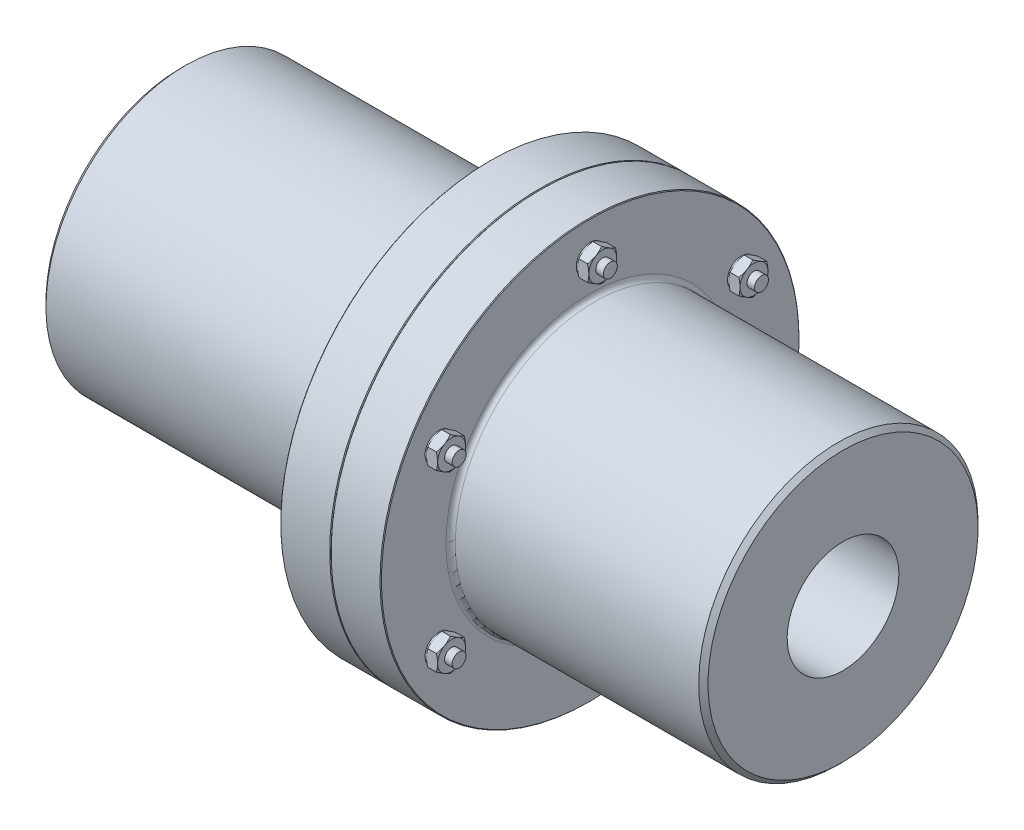
from build123d import *

# Parameters (mm, degrees)
CHAMFER1_SIZE                   = 3.333333333
CHAMFER2_SIZE                   = 0.5
FILLET1_R                       = 1
SKETCH15_R                      = 65
CUT_EXTRUDE5_DEPTH              = 334.240153643
CUT_EXTRUDE7_DEPTH              = 334.240153643
SKETCH16_R                      = 60
CUT_EXTRUDE6_DEPTH              = 334.240153643
CHAMFER3_SIZE                   = 0.5
CHAMFER4_SIZE                   = 3.333333333
FILLET2_R                       = 3.333333333
SKETCH6_R                       = 5
CUT_EXTRUDE1_DEPTH              = 72
CHAMFER5_SIZE                   = 0.2
CHAMFER6_SIZE                   = 0.2
CIRCPATTERN1_COUNT              = 6
CHAMFER5_OF_CIRCPATTERN1_SIZE   = 0.2
CHAMFER6_OF_CIRCPATTERN1_SIZE   = 0.2
SKETCH7_W                       = 86.4
SKETCH7_H                       = 5
BOSS_EXTRUDE1_DEPTH             = 8
SKETCH9_R                       = 15
SKETCH9_R_2                     = 10
CUT_EXTRUDE2_DEPTH              = 1
CUT_EXTRUDE2_DRAFT              = -60
SKETCH10_R                      = 10
BOSS_EXTRUDE2_DEPTH             = 1
BOSS_EXTRUDE3_DEPTH             = 8
SKETCH12_R                      = 15
SKETCH12_R_2                    = 10
CUT_EXTRUDE3_DEPTH              = 1
CUT_EXTRUDE3_DRAFT              = -60
SKETCH13_R                      = 15
SKETCH13_R_2                    = 10
CUT_EXTRUDE4_DEPTH              = 1
CUT_EXTRUDE4_DRAFT              = -60
CIRCPATTERN3_COUNT              = 6
CIRCPATTERN3_COPY_1_SKETCH_R    = 15
CIRCPATTERN3_COPY_1_SKETCH_R_2  = 10
CIRCPATTERN3_COPY_1_DEPTH       = 1
CIRCPATTERN3_COPY_1_DRAFT       = -60
CIRCPATTERN3_COPY_2_SKETCH_R    = 15
CIRCPATTERN3_COPY_2_SKETCH_R_2  = 10
CIRCPATTERN3_COPY_2_DEPTH       = 1
CIRCPATTERN3_COPY_2_DRAFT       = -60
CIRCPATTERN3_COPY_3_SKETCH_R    = 15
CIRCPATTERN3_COPY_3_SKETCH_R_2  = 10
CIRCPATTERN3_COPY_3_DEPTH       = 1
CIRCPATTERN3_COPY_3_DRAFT       = -60
CIRCPATTERN3_COPY_4_SKETCH_R    = 15
CIRCPATTERN3_COPY_4_SKETCH_R_2  = 10
CIRCPATTERN3_COPY_4_DEPTH       = 1
CIRCPATTERN3_COPY_4_DRAFT       = -60
CIRCPATTERN3_COPY_5_SKETCH_R    = 15
CIRCPATTERN3_COPY_5_SKETCH_R_2  = 10
CIRCPATTERN3_COPY_5_DEPTH       = 1
CIRCPATTERN3_COPY_5_DRAFT       = -60
CIRCPATTERN3_COPY_6_SKETCH_R    = 15
CIRCPATTERN3_COPY_6_SKETCH_R_2  = 10
CIRCPATTERN3_COPY_6_DEPTH       = 1
CIRCPATTERN3_COPY_6_DRAFT       = -60
CIRCPATTERN3_COPY_7_SKETCH_R    = 15
CIRCPATTERN3_COPY_7_SKETCH_R_2  = 10
CIRCPATTERN3_COPY_7_DEPTH       = 1
CIRCPATTERN3_COPY_7_DRAFT       = -60
CIRCPATTERN3_COPY_8_SKETCH_R    = 15
CIRCPATTERN3_COPY_8_SKETCH_R_2  = 10
CIRCPATTERN3_COPY_8_DEPTH       = 1
CIRCPATTERN3_COPY_8_DRAFT       = -60
CIRCPATTERN3_COPY_9_SKETCH_R    = 15
CIRCPATTERN3_COPY_9_SKETCH_R_2  = 10
CIRCPATTERN3_COPY_9_DEPTH       = 1
CIRCPATTERN3_COPY_9_DRAFT       = -60
CIRCPATTERN3_COPY_10_SKETCH_R   = 15
CIRCPATTERN3_COPY_10_SKETCH_R_2 = 10
CIRCPATTERN3_COPY_10_DEPTH      = 1
CIRCPATTERN3_COPY_10_DRAFT      = -60
CIRCPATTERN3_COPY_11_SKETCH_R   = 15
CIRCPATTERN3_COPY_11_SKETCH_R_2 = 10
CIRCPATTERN3_COPY_11_DEPTH      = 1
CIRCPATTERN3_COPY_11_DRAFT      = -60
CIRCPATTERN3_COPY_12_SKETCH_R   = 15
CIRCPATTERN3_COPY_12_SKETCH_R_2 = 10
CIRCPATTERN3_COPY_12_DEPTH      = 1
CIRCPATTERN3_COPY_12_DRAFT      = -60
CIRCPATTERN3_COPY_13_SKETCH_R   = 15
CIRCPATTERN3_COPY_13_SKETCH_R_2 = 10
CIRCPATTERN3_COPY_13_DEPTH      = 1
CIRCPATTERN3_COPY_13_DRAFT      = -60
CIRCPATTERN3_COPY_14_SKETCH_R   = 15
CIRCPATTERN3_COPY_14_SKETCH_R_2 = 10
CIRCPATTERN3_COPY_14_DEPTH      = 1
CIRCPATTERN3_COPY_14_DRAFT      = -60
CIRCPATTERN3_COPY_15_SKETCH_R   = 15
CIRCPATTERN3_COPY_15_SKETCH_R_2 = 10
CIRCPATTERN3_COPY_15_DEPTH      = 1
CIRCPATTERN3_COPY_15_DRAFT      = -60
SKETCH27_R                      = 60
SKETCH27_R_2                    = 40
BOSS_EXTRUDE4_DEPTH             = 212


with BuildPart() as part:
    # Sketch2 → Revolve1 (revolve)
    with BuildSketch(Plane.XY, mode=Mode.PRIVATE) as revolve1_sk:
        Polygon((-257, 100), (-257, 0), (-5, 0), (-5, 105), (0, 105), (0, 150), (-36, 150), (-36, 100), align=None)
    revolve(revolve1_sk.sketch.rotate(Axis((-257, 0, 0), (1, 0, 0)), 180), axis=Axis((-257, 0, 0), (1, 0, 0)))

    # Chamfer1
    chamfer1_edges = [part.edges().sort_by_distance(p)[0] for p in [
        (-257, 100, 0),
    ]]
    chamfer(chamfer1_edges, length=CHAMFER1_SIZE)

    # Chamfer2
    chamfer2_edges = [part.edges().sort_by_distance(p)[0] for p in [
        (-36, 150, 0),
        (0, 150, 0),
    ]]
    chamfer(chamfer2_edges, length=CHAMFER2_SIZE)

    # Fillet1
    fillet1_edges = [part.edges().sort_by_distance(p)[0] for p in [
        (-36, 100, 0),
    ]]
    fillet(fillet1_edges, radius=FILLET1_R)

    # Sketch15 → Cut-Extrude5 (cut, through all)
    with BuildSketch(Plane(origin=(0, 0, 0), x_dir=(0, 0, -1), z_dir=(1, 0, 0))):
        Circle(SKETCH15_R)
    extrude(amount=-CUT_EXTRUDE5_DEPTH, mode=Mode.SUBTRACT)

    # Sketch20 → Cut-Extrude7 (cut, through all)
    with BuildSketch(Plane(origin=(0, 0, 0), x_dir=(0, 0, -1), z_dir=(1, 0, 0))):
        with BuildLine():
            Line((72.4, -16), (72.4, 16))
            Line((72.4, 16), (63, 16))
            ThreePointArc((63, 16), (64.498061986, 8.062257748), (65, 0))
            ThreePointArc((65, 0), (64.498061986, -8.062257748), (63, -16))
            Line((63, -16), (72.4, -16))
        make_face()
    extrude(amount=-CUT_EXTRUDE7_DEPTH, mode=Mode.SUBTRACT)


with BuildPart() as body_2:
    # Sketch3 → Revolve2 (revolve)
    with BuildSketch(Plane.XY):
        Polygon((36, 150), (0, 150), (0, 105), (5, 105), (5, 0), (217, 0), (217, 60), (217, 100), (36, 100), align=None)
    revolve(axis=Axis((-257, 0, 0), (1, 0, 0)))

    # Sketch16 → Cut-Extrude6 (cut, through all)
    with BuildSketch(Plane(origin=(0, 0, 0), x_dir=(0, 0, -1), z_dir=(1, 0, 0))):
        with Locations(Location((0, 0, 0), (0, 0, 90))):
            Circle(SKETCH16_R)
    extrude(amount=CUT_EXTRUDE6_DEPTH, mode=Mode.SUBTRACT)

    # Chamfer3
    chamfer3_edges = [body_2.edges().sort_by_distance(p)[0] for p in [
        (36, -150, 0),
        (0, -150, 0),
    ]]
    chamfer(chamfer3_edges, length=CHAMFER3_SIZE)

    # Chamfer4
    chamfer4_edges = [body_2.edges().sort_by_distance(p)[0] for p in [
        (217, -100, 0),
    ]]
    chamfer(chamfer4_edges, length=CHAMFER4_SIZE)

    # Fillet2
    fillet2_edges = [body_2.edges().sort_by_distance(p)[0] for p in [
        (36, -100, 0),
    ]]
    fillet(fillet2_edges, radius=FILLET2_R)


with BuildPart() as cut_extrude1_tool:
    # Sketch6 → Cut-Extrude1 (new body)
    with BuildSketch(Plane.ZY.offset(36)):
        with Locations((0, 125)):
            Circle(SKETCH6_R)
    cut_extrude1 = extrude(amount=-CUT_EXTRUDE1_DEPTH)


with BuildPart() as part_1:
    add(part.part)

    # Cut-Extrude1: cut by cut_extrude1_tool
    add(cut_extrude1_tool.part, mode=Mode.SUBTRACT)

    # Chamfer5
    chamfer5_edges = [part_1.edges().sort_by_distance(p)[0] for p in [
        (-36, 125, -5),
    ]]
    chamfer(chamfer5_edges, length=CHAMFER5_SIZE)


with BuildPart() as body_2_1:
    add(body_2.part)

    # Cut-Extrude1: cut by cut_extrude1_tool
    add(cut_extrude1_tool.part, mode=Mode.SUBTRACT)

    # Chamfer6
    chamfer6_edges = [body_2_1.edges().sort_by_distance(p)[0] for p in [
        (36, 125, -5),
    ]]
    chamfer(chamfer6_edges, length=CHAMFER6_SIZE)


with BuildPart() as circpattern1_tool:
    # CircPattern1: Cut-Extrude1 ×6 about axis
    circpattern1_axis = Axis((0, 0, 0), (1, 0, 0))
    for i in range(1, CIRCPATTERN1_COUNT):
        add(cut_extrude1.rotate(circpattern1_axis, i * 360 / CIRCPATTERN1_COUNT))


with BuildPart() as part_2:
    add(part_1.part)

    # CircPattern1: cut by circpattern1_tool
    add(circpattern1_tool.part, mode=Mode.SUBTRACT)

    # Chamfer5 of CircPattern1
    chamfer5_of_circpattern1_edges = [part_2.edges().sort_by_distance(p)[0] for p in [
        (-36, 66.830127019, 105.753175473),
        (-36, -58.169872981, 110.753175473),
        (-36, -125, 5),
        (-36, -66.830127019, -105.753175473),
        (-36, 58.169872981, -110.753175473),
    ]]
    chamfer(chamfer5_of_circpattern1_edges, length=CHAMFER5_OF_CIRCPATTERN1_SIZE)



with BuildPart() as body_2_2:
    add(body_2_1.part)

    # CircPattern1: cut by circpattern1_tool
    add(circpattern1_tool.part, mode=Mode.SUBTRACT)

    # Chamfer6 of CircPattern1
    chamfer6_of_circpattern1_edges = [body_2_2.edges().sort_by_distance(p)[0] for p in [
        (36, 66.830127019, 105.753175473),
        (36, -58.169872981, 110.753175473),
        (36, -125, 5),
        (36, -66.830127019, -105.753175473),
        (36, 58.169872981, -110.753175473),
    ]]
    chamfer(chamfer6_of_circpattern1_edges, length=CHAMFER6_OF_CIRCPATTERN1_SIZE)


with BuildPart() as part_3:
    add(part_2.part)

    add(body_2_2.part)  # Revolve3 merges body 2
    # Sketch7 → Revolve3 (revolve)
    with BuildSketch(Plane.XY, mode=Mode.PRIVATE) as revolve3_sk:
        with Locations((7.2, 127.5)):
            Rectangle(SKETCH7_W, SKETCH7_H)
    revolve3 = revolve(revolve3_sk.sketch.rotate(Axis((50.4, 125, 0), (-1, 0, 0)), 90), axis=Axis((50.4, 125, 0), (-1, 0, 0)))

    # Sketch8 → Boss-Extrude1 (add)
    with BuildSketch(Plane.ZY.offset(36)):
        Polygon((0, 136.547005384), (-10, 130.773502692), (-10, 119.226497308), (0, 113.452994616), (10, 119.226497308), (10, 130.773502692), align=None)
    boss_extrude1 = extrude(amount=BOSS_EXTRUDE1_DEPTH)


with BuildPart() as cut_extrude2_tool:
    # Sketch9 → Cut-Extrude2 (with draft: the straight prism first)
    with BuildSketch(Plane.ZY.offset(44)):
        with Locations((0, 125)):
            Circle(SKETCH9_R)
        with Locations((0, 125)):
            Circle(SKETCH9_R_2, mode=Mode.SUBTRACT)
    extrude(amount=-CUT_EXTRUDE2_DEPTH)
    # Cut-Extrude2: the draft: its side faces are tilted about the plane it starts from
    cut_extrude2_sides = [cut_extrude2_tool.faces().sort_by_distance(p)[0] for p in [
        (-43.5, 125, -15),
        (-43.5, 125, -10),
    ]]
    draft(cut_extrude2_sides, Plane.ZY.offset(44), CUT_EXTRUDE2_DRAFT)


with BuildPart() as part_4:
    add(part_3.part)

    # Cut-Extrude2: cut by cut_extrude2_tool
    add(cut_extrude2_tool.part, mode=Mode.SUBTRACT)

    # Sketch10 → Boss-Extrude2 (add)
    with BuildSketch(Plane(origin=(36, 0, 0), x_dir=(0, 0, -1), z_dir=(1, 0, 0))):
        with Locations(Location((0, 125, 0), (0, 0, 270))):
            Circle(SKETCH10_R)
    boss_extrude2 = extrude(amount=BOSS_EXTRUDE2_DEPTH)

    # Sketch11 → Boss-Extrude3 (add)
    with BuildSketch(Plane(origin=(37, 0, 0), x_dir=(0, 0, -1), z_dir=(1, 0, 0))):
        Polygon((10, 130.773502692), (0, 136.547005384), (-10, 130.773502692), (-10, 119.226497308), (0, 113.452994616), (10, 119.226497308), align=None)
    boss_extrude3 = extrude(amount=BOSS_EXTRUDE3_DEPTH)


with BuildPart() as cut_extrude3_tool:
    # Sketch12 → Cut-Extrude3 (with draft: the straight prism first)
    with BuildSketch(Plane(origin=(45, 0, 0), x_dir=(0, 0, -1), z_dir=(1, 0, 0))):
        with Locations((0, 125)):
            Circle(SKETCH12_R)
        with Locations(Location((0, 125, 0), (0, 0, 180))):
            Circle(SKETCH12_R_2, mode=Mode.SUBTRACT)
    extrude(amount=-CUT_EXTRUDE3_DEPTH)
    # Cut-Extrude3: the draft: its side faces are tilted about the plane it starts from
    cut_extrude3_sides = [cut_extrude3_tool.faces().sort_by_distance(p)[0] for p in [
        (44.5, 125, 15),
        (44.5, 125, -10),
    ]]
    draft(cut_extrude3_sides, Plane(origin=(45, 0, 0), x_dir=(0, 0, -1), z_dir=(1, 0, 0)), CUT_EXTRUDE3_DRAFT)


with BuildPart() as part_5:
    add(part_4.part)

    # Cut-Extrude3: cut by cut_extrude3_tool
    add(cut_extrude3_tool.part, mode=Mode.SUBTRACT)


with BuildPart() as cut_extrude4_tool:
    # Sketch13 → Cut-Extrude4 (with draft: the straight prism first)
    with BuildSketch(Plane.ZY.offset(-37)):
        with Locations((0, 125)):
            Circle(SKETCH13_R)
        with Locations((0, 125)):
            Circle(SKETCH13_R_2, mode=Mode.SUBTRACT)
    extrude(amount=-CUT_EXTRUDE4_DEPTH)
    # Cut-Extrude4: the draft: its side faces are tilted about the plane it starts from
    cut_extrude4_sides = [cut_extrude4_tool.faces().sort_by_distance(p)[0] for p in [
        (37.5, 125, -15),
        (37.5, 125, -10),
    ]]
    draft(cut_extrude4_sides, Plane.ZY.offset(-37), CUT_EXTRUDE4_DRAFT)


with BuildPart() as part_6:
    add(part_5.part)

    # Cut-Extrude4: cut by cut_extrude4_tool
    add(cut_extrude4_tool.part, mode=Mode.SUBTRACT)

    # CircPattern3: Revolve3, Boss-Extrude1, Boss-Extrude2, Boss-Extrude3 ×6 about axis
    circpattern3_axis = Axis((0, 0, 0), (1, 0, 0))
    add([revolve3.rotate(circpattern3_axis, i * 360 / CIRCPATTERN3_COUNT) for i in range(1, CIRCPATTERN3_COUNT)])
    add([boss_extrude1.rotate(circpattern3_axis, i * 360 / CIRCPATTERN3_COUNT) for i in range(1, CIRCPATTERN3_COUNT)])
    add([boss_extrude2.rotate(circpattern3_axis, i * 360 / CIRCPATTERN3_COUNT) for i in range(1, CIRCPATTERN3_COUNT)])
    add([boss_extrude3.rotate(circpattern3_axis, i * 360 / CIRCPATTERN3_COUNT) for i in range(1, CIRCPATTERN3_COUNT)])


with BuildPart() as circpattern3_copy_1_tool:
    # CircPattern3 copy 1 sketch → CircPattern3 copy 1 (with draft: the straight prism first)
    with BuildSketch(Plane(origin=(-44, 0, 0), x_dir=(0, -0.8660254037844386, 0.5000000000000001), z_dir=(-1, 0, 0))):
        with Locations((0, 125)):
            Circle(CIRCPATTERN3_COPY_1_SKETCH_R)
        with Locations((0, 125)):
            Circle(CIRCPATTERN3_COPY_1_SKETCH_R_2, mode=Mode.SUBTRACT)
    extrude(amount=-CIRCPATTERN3_COPY_1_DEPTH)
    # CircPattern3 copy 1: the draft: its side faces are tilted about the plane it starts from
    circpattern3_copy_1_sides = [circpattern3_copy_1_tool.faces().sort_by_distance(p)[0] for p in [
        (-43.5, 75.490381057, 100.753175473),
        (-43.5, 71.160254038, 103.253175473),
    ]]
    draft(circpattern3_copy_1_sides, Plane(origin=(-44, 0, 0), x_dir=(0, -0.8660254037844386, 0.5000000000000001), z_dir=(-1, 0, 0)), CIRCPATTERN3_COPY_1_DRAFT)


with BuildPart() as part_7:
    add(part_6.part)

    # CircPattern3 copy 1: cut by circpattern3_copy_1_tool
    add(circpattern3_copy_1_tool.part, mode=Mode.SUBTRACT)


with BuildPart() as circpattern3_copy_2_tool:
    # CircPattern3 copy 2 sketch → CircPattern3 copy 2 (with draft: the straight prism first)
    with BuildSketch(Plane(origin=(-44, 0, 0), x_dir=(0, -0.8660254037844387, -0.4999999999999998), z_dir=(-1, 0, 0))):
        with Locations((0, 125)):
            Circle(CIRCPATTERN3_COPY_2_SKETCH_R)
        with Locations((0, 125)):
            Circle(CIRCPATTERN3_COPY_2_SKETCH_R_2, mode=Mode.SUBTRACT)
    extrude(amount=-CIRCPATTERN3_COPY_2_DEPTH)
    # CircPattern3 copy 2: the draft: its side faces are tilted about the plane it starts from
    circpattern3_copy_2_sides = [circpattern3_copy_2_tool.faces().sort_by_distance(p)[0] for p in [
        (-43.5, -49.509618943, 115.753175473),
        (-43.5, -53.839745962, 113.253175473),
    ]]
    draft(circpattern3_copy_2_sides, Plane(origin=(-44, 0, 0), x_dir=(0, -0.8660254037844387, -0.4999999999999998), z_dir=(-1, 0, 0)), CIRCPATTERN3_COPY_2_DRAFT)


with BuildPart() as part_8:
    add(part_7.part)

    # CircPattern3 copy 2: cut by circpattern3_copy_2_tool
    add(circpattern3_copy_2_tool.part, mode=Mode.SUBTRACT)


with BuildPart() as circpattern3_copy_3_tool:
    # CircPattern3 copy 3 sketch → CircPattern3 copy 3 (with draft: the straight prism first)
    with BuildSketch(Plane(origin=(-44, 0, 0), x_dir=(0, 0, -1), z_dir=(-1, 0, 0))):
        with Locations((0, 125)):
            Circle(CIRCPATTERN3_COPY_3_SKETCH_R)
        with Locations((0, 125)):
            Circle(CIRCPATTERN3_COPY_3_SKETCH_R_2, mode=Mode.SUBTRACT)
    extrude(amount=-CIRCPATTERN3_COPY_3_DEPTH)
    # CircPattern3 copy 3: the draft: its side faces are tilted about the plane it starts from
    circpattern3_copy_3_sides = [circpattern3_copy_3_tool.faces().sort_by_distance(p)[0] for p in [
        (-43.5, -125, 15),
        (-43.5, -125, 10),
    ]]
    draft(circpattern3_copy_3_sides, Plane(origin=(-44, 0, 0), x_dir=(0, 0, -1), z_dir=(-1, 0, 0)), CIRCPATTERN3_COPY_3_DRAFT)


with BuildPart() as part_9:
    add(part_8.part)

    # CircPattern3 copy 3: cut by circpattern3_copy_3_tool
    add(circpattern3_copy_3_tool.part, mode=Mode.SUBTRACT)


with BuildPart() as circpattern3_copy_4_tool:
    # CircPattern3 copy 4 sketch → CircPattern3 copy 4 (with draft: the straight prism first)
    with BuildSketch(Plane(origin=(-44, 0, 0), x_dir=(0, 0.8660254037844384, -0.5000000000000004), z_dir=(-1, 0, 0))):
        with Locations((0, 125)):
            Circle(CIRCPATTERN3_COPY_4_SKETCH_R)
        with Locations((0, 125)):
            Circle(CIRCPATTERN3_COPY_4_SKETCH_R_2, mode=Mode.SUBTRACT)
    extrude(amount=-CIRCPATTERN3_COPY_4_DEPTH)
    # CircPattern3 copy 4: the draft: its side faces are tilted about the plane it starts from
    circpattern3_copy_4_sides = [circpattern3_copy_4_tool.faces().sort_by_distance(p)[0] for p in [
        (-43.5, -75.490381057, -100.753175473),
        (-43.5, -71.160254038, -103.253175473),
    ]]
    draft(circpattern3_copy_4_sides, Plane(origin=(-44, 0, 0), x_dir=(0, 0.8660254037844384, -0.5000000000000004), z_dir=(-1, 0, 0)), CIRCPATTERN3_COPY_4_DRAFT)


with BuildPart() as part_10:
    add(part_9.part)

    # CircPattern3 copy 4: cut by circpattern3_copy_4_tool
    add(circpattern3_copy_4_tool.part, mode=Mode.SUBTRACT)


with BuildPart() as circpattern3_copy_5_tool:
    # CircPattern3 copy 5 sketch → CircPattern3 copy 5 (with draft: the straight prism first)
    with BuildSketch(Plane(origin=(-44, 0, 0), x_dir=(0, 0.8660254037844386, 0.5000000000000001), z_dir=(-1, 0, 0))):
        with Locations((0, 125)):
            Circle(CIRCPATTERN3_COPY_5_SKETCH_R)
        with Locations((0, 125)):
            Circle(CIRCPATTERN3_COPY_5_SKETCH_R_2, mode=Mode.SUBTRACT)
    extrude(amount=-CIRCPATTERN3_COPY_5_DEPTH)
    # CircPattern3 copy 5: the draft: its side faces are tilted about the plane it starts from
    circpattern3_copy_5_sides = [circpattern3_copy_5_tool.faces().sort_by_distance(p)[0] for p in [
        (-43.5, 49.509618943, -115.753175473),
        (-43.5, 53.839745962, -113.253175473),
    ]]
    draft(circpattern3_copy_5_sides, Plane(origin=(-44, 0, 0), x_dir=(0, 0.8660254037844386, 0.5000000000000001), z_dir=(-1, 0, 0)), CIRCPATTERN3_COPY_5_DRAFT)


with BuildPart() as part_11:
    add(part_10.part)

    # CircPattern3 copy 5: cut by circpattern3_copy_5_tool
    add(circpattern3_copy_5_tool.part, mode=Mode.SUBTRACT)


with BuildPart() as circpattern3_copy_6_tool:
    # CircPattern3 copy 6 sketch → CircPattern3 copy 6 (with draft: the straight prism first)
    with BuildSketch(Plane(origin=(45, 0, 0), x_dir=(0, 0.8660254037844386, -0.5000000000000001), z_dir=(1, 0, 0))):
        with Locations((0, 125)):
            Circle(CIRCPATTERN3_COPY_6_SKETCH_R)
        with Locations(Location((0, 125, 0), (0, 0, 180))):
            Circle(CIRCPATTERN3_COPY_6_SKETCH_R_2, mode=Mode.SUBTRACT)
    extrude(amount=-CIRCPATTERN3_COPY_6_DEPTH)
    # CircPattern3 copy 6: the draft: its side faces are tilted about the plane it starts from
    circpattern3_copy_6_sides = [circpattern3_copy_6_tool.faces().sort_by_distance(p)[0] for p in [
        (44.5, 49.509618943, 115.753175473),
        (44.5, 71.160254038, 103.253175473),
    ]]
    draft(circpattern3_copy_6_sides, Plane(origin=(45, 0, 0), x_dir=(0, 0.8660254037844386, -0.5000000000000001), z_dir=(1, 0, 0)), CIRCPATTERN3_COPY_6_DRAFT)


with BuildPart() as part_12:
    add(part_11.part)

    # CircPattern3 copy 6: cut by circpattern3_copy_6_tool
    add(circpattern3_copy_6_tool.part, mode=Mode.SUBTRACT)


with BuildPart() as circpattern3_copy_7_tool:
    # CircPattern3 copy 7 sketch → CircPattern3 copy 7 (with draft: the straight prism first)
    with BuildSketch(Plane(origin=(45, 0, 0), x_dir=(0, 0.8660254037844387, 0.4999999999999998), z_dir=(1, 0, 0))):
        with Locations((0, 125)):
            Circle(CIRCPATTERN3_COPY_7_SKETCH_R)
        with Locations(Location((0, 125, 0), (0, 0, 180))):
            Circle(CIRCPATTERN3_COPY_7_SKETCH_R_2, mode=Mode.SUBTRACT)
    extrude(amount=-CIRCPATTERN3_COPY_7_DEPTH)
    # CircPattern3 copy 7: the draft: its side faces are tilted about the plane it starts from
    circpattern3_copy_7_sides = [circpattern3_copy_7_tool.faces().sort_by_distance(p)[0] for p in [
        (44.5, -75.490381057, 100.753175473),
        (44.5, -53.839745962, 113.253175473),
    ]]
    draft(circpattern3_copy_7_sides, Plane(origin=(45, 0, 0), x_dir=(0, 0.8660254037844387, 0.4999999999999998), z_dir=(1, 0, 0)), CIRCPATTERN3_COPY_7_DRAFT)


with BuildPart() as part_13:
    add(part_12.part)

    # CircPattern3 copy 7: cut by circpattern3_copy_7_tool
    add(circpattern3_copy_7_tool.part, mode=Mode.SUBTRACT)


with BuildPart() as circpattern3_copy_8_tool:
    # CircPattern3 copy 8 sketch → CircPattern3 copy 8 (with draft: the straight prism first)
    with BuildSketch(Plane(origin=(45, 0, 0), x_dir=(0, 0, 1), z_dir=(1, 0, 0))):
        with Locations((0, 125)):
            Circle(CIRCPATTERN3_COPY_8_SKETCH_R)
        with Locations(Location((0, 125, 0), (0, 0, 180))):
            Circle(CIRCPATTERN3_COPY_8_SKETCH_R_2, mode=Mode.SUBTRACT)
    extrude(amount=-CIRCPATTERN3_COPY_8_DEPTH)
    # CircPattern3 copy 8: the draft: its side faces are tilted about the plane it starts from
    circpattern3_copy_8_sides = [circpattern3_copy_8_tool.faces().sort_by_distance(p)[0] for p in [
        (44.5, -125, -15),
        (44.5, -125, 10),
    ]]
    draft(circpattern3_copy_8_sides, Plane(origin=(45, 0, 0), x_dir=(0, 0, 1), z_dir=(1, 0, 0)), CIRCPATTERN3_COPY_8_DRAFT)


with BuildPart() as part_14:
    add(part_13.part)

    # CircPattern3 copy 8: cut by circpattern3_copy_8_tool
    add(circpattern3_copy_8_tool.part, mode=Mode.SUBTRACT)


with BuildPart() as circpattern3_copy_9_tool:
    # CircPattern3 copy 9 sketch → CircPattern3 copy 9 (with draft: the straight prism first)
    with BuildSketch(Plane(origin=(45, 0, 0), x_dir=(0, -0.8660254037844384, 0.5000000000000004), z_dir=(1, 0, 0))):
        with Locations((0, 125)):
            Circle(CIRCPATTERN3_COPY_9_SKETCH_R)
        with Locations(Location((0, 125, 0), (0, 0, 180))):
            Circle(CIRCPATTERN3_COPY_9_SKETCH_R_2, mode=Mode.SUBTRACT)
    extrude(amount=-CIRCPATTERN3_COPY_9_DEPTH)
    # CircPattern3 copy 9: the draft: its side faces are tilted about the plane it starts from
    circpattern3_copy_9_sides = [circpattern3_copy_9_tool.faces().sort_by_distance(p)[0] for p in [
        (44.5, -49.509618943, -115.753175473),
        (44.5, -71.160254038, -103.253175473),
    ]]
    draft(circpattern3_copy_9_sides, Plane(origin=(45, 0, 0), x_dir=(0, -0.8660254037844384, 0.5000000000000004), z_dir=(1, 0, 0)), CIRCPATTERN3_COPY_9_DRAFT)


with BuildPart() as part_15:
    add(part_14.part)

    # CircPattern3 copy 9: cut by circpattern3_copy_9_tool
    add(circpattern3_copy_9_tool.part, mode=Mode.SUBTRACT)


with BuildPart() as circpattern3_copy_10_tool:
    # CircPattern3 copy 10 sketch → CircPattern3 copy 10 (with draft: the straight prism first)
    with BuildSketch(Plane(origin=(45, 0, 0), x_dir=(0, -0.8660254037844386, -0.5000000000000001), z_dir=(1, 0, 0))):
        with Locations((0, 125)):
            Circle(CIRCPATTERN3_COPY_10_SKETCH_R)
        with Locations(Location((0, 125, 0), (0, 0, 180))):
            Circle(CIRCPATTERN3_COPY_10_SKETCH_R_2, mode=Mode.SUBTRACT)
    extrude(amount=-CIRCPATTERN3_COPY_10_DEPTH)
    # CircPattern3 copy 10: the draft: its side faces are tilted about the plane it starts from
    circpattern3_copy_10_sides = [circpattern3_copy_10_tool.faces().sort_by_distance(p)[0] for p in [
        (44.5, 75.490381057, -100.753175473),
        (44.5, 53.839745962, -113.253175473),
    ]]
    draft(circpattern3_copy_10_sides, Plane(origin=(45, 0, 0), x_dir=(0, -0.8660254037844386, -0.5000000000000001), z_dir=(1, 0, 0)), CIRCPATTERN3_COPY_10_DRAFT)


with BuildPart() as part_16:
    add(part_15.part)

    # CircPattern3 copy 10: cut by circpattern3_copy_10_tool
    add(circpattern3_copy_10_tool.part, mode=Mode.SUBTRACT)


with BuildPart() as circpattern3_copy_11_tool:
    # CircPattern3 copy 11 sketch → CircPattern3 copy 11 (with draft: the straight prism first)
    with BuildSketch(Plane(origin=(37, 0, 0), x_dir=(0, -0.8660254037844386, 0.5000000000000001), z_dir=(-1, 0, 0))):
        with Locations((0, 125)):
            Circle(CIRCPATTERN3_COPY_11_SKETCH_R)
        with Locations((0, 125)):
            Circle(CIRCPATTERN3_COPY_11_SKETCH_R_2, mode=Mode.SUBTRACT)
    extrude(amount=-CIRCPATTERN3_COPY_11_DEPTH)
    # CircPattern3 copy 11: the draft: its side faces are tilted about the plane it starts from
    circpattern3_copy_11_sides = [circpattern3_copy_11_tool.faces().sort_by_distance(p)[0] for p in [
        (37.5, 75.490381057, 100.753175473),
        (37.5, 71.160254038, 103.253175473),
    ]]
    draft(circpattern3_copy_11_sides, Plane(origin=(37, 0, 0), x_dir=(0, -0.8660254037844386, 0.5000000000000001), z_dir=(-1, 0, 0)), CIRCPATTERN3_COPY_11_DRAFT)


with BuildPart() as part_17:
    add(part_16.part)

    # CircPattern3 copy 11: cut by circpattern3_copy_11_tool
    add(circpattern3_copy_11_tool.part, mode=Mode.SUBTRACT)


with BuildPart() as circpattern3_copy_12_tool:
    # CircPattern3 copy 12 sketch → CircPattern3 copy 12 (with draft: the straight prism first)
    with BuildSketch(Plane(origin=(37, 0, 0), x_dir=(0, -0.8660254037844387, -0.4999999999999998), z_dir=(-1, 0, 0))):
        with Locations((0, 125)):
            Circle(CIRCPATTERN3_COPY_12_SKETCH_R)
        with Locations((0, 125)):
            Circle(CIRCPATTERN3_COPY_12_SKETCH_R_2, mode=Mode.SUBTRACT)
    extrude(amount=-CIRCPATTERN3_COPY_12_DEPTH)
    # CircPattern3 copy 12: the draft: its side faces are tilted about the plane it starts from
    circpattern3_copy_12_sides = [circpattern3_copy_12_tool.faces().sort_by_distance(p)[0] for p in [
        (37.5, -49.509618943, 115.753175473),
        (37.5, -53.839745962, 113.253175473),
    ]]
    draft(circpattern3_copy_12_sides, Plane(origin=(37, 0, 0), x_dir=(0, -0.8660254037844387, -0.4999999999999998), z_dir=(-1, 0, 0)), CIRCPATTERN3_COPY_12_DRAFT)


with BuildPart() as part_18:
    add(part_17.part)

    # CircPattern3 copy 12: cut by circpattern3_copy_12_tool
    add(circpattern3_copy_12_tool.part, mode=Mode.SUBTRACT)


with BuildPart() as circpattern3_copy_13_tool:
    # CircPattern3 copy 13 sketch → CircPattern3 copy 13 (with draft: the straight prism first)
    with BuildSketch(Plane(origin=(37, 0, 0), x_dir=(0, 0, -1), z_dir=(-1, 0, 0))):
        with Locations((0, 125)):
            Circle(CIRCPATTERN3_COPY_13_SKETCH_R)
        with Locations((0, 125)):
            Circle(CIRCPATTERN3_COPY_13_SKETCH_R_2, mode=Mode.SUBTRACT)
    extrude(amount=-CIRCPATTERN3_COPY_13_DEPTH)
    # CircPattern3 copy 13: the draft: its side faces are tilted about the plane it starts from
    circpattern3_copy_13_sides = [circpattern3_copy_13_tool.faces().sort_by_distance(p)[0] for p in [
        (37.5, -125, 15),
        (37.5, -125, 10),
    ]]
    draft(circpattern3_copy_13_sides, Plane(origin=(37, 0, 0), x_dir=(0, 0, -1), z_dir=(-1, 0, 0)), CIRCPATTERN3_COPY_13_DRAFT)


with BuildPart() as part_19:
    add(part_18.part)

    # CircPattern3 copy 13: cut by circpattern3_copy_13_tool
    add(circpattern3_copy_13_tool.part, mode=Mode.SUBTRACT)


with BuildPart() as circpattern3_copy_14_tool:
    # CircPattern3 copy 14 sketch → CircPattern3 copy 14 (with draft: the straight prism first)
    with BuildSketch(Plane(origin=(37, 0, 0), x_dir=(0, 0.8660254037844384, -0.5000000000000004), z_dir=(-1, 0, 0))):
        with Locations((0, 125)):
            Circle(CIRCPATTERN3_COPY_14_SKETCH_R)
        with Locations((0, 125)):
            Circle(CIRCPATTERN3_COPY_14_SKETCH_R_2, mode=Mode.SUBTRACT)
    extrude(amount=-CIRCPATTERN3_COPY_14_DEPTH)
    # CircPattern3 copy 14: the draft: its side faces are tilted about the plane it starts from
    circpattern3_copy_14_sides = [circpattern3_copy_14_tool.faces().sort_by_distance(p)[0] for p in [
        (37.5, -75.490381057, -100.753175473),
        (37.5, -71.160254038, -103.253175473),
    ]]
    draft(circpattern3_copy_14_sides, Plane(origin=(37, 0, 0), x_dir=(0, 0.8660254037844384, -0.5000000000000004), z_dir=(-1, 0, 0)), CIRCPATTERN3_COPY_14_DRAFT)


with BuildPart() as part_20:
    add(part_19.part)

    # CircPattern3 copy 14: cut by circpattern3_copy_14_tool
    add(circpattern3_copy_14_tool.part, mode=Mode.SUBTRACT)


with BuildPart() as circpattern3_copy_15_tool:
    # CircPattern3 copy 15 sketch → CircPattern3 copy 15 (with draft: the straight prism first)
    with BuildSketch(Plane(origin=(37, 0, 0), x_dir=(0, 0.8660254037844386, 0.5000000000000001), z_dir=(-1, 0, 0))):
        with Locations((0, 125)):
            Circle(CIRCPATTERN3_COPY_15_SKETCH_R)
        with Locations((0, 125)):
            Circle(CIRCPATTERN3_COPY_15_SKETCH_R_2, mode=Mode.SUBTRACT)
    extrude(amount=-CIRCPATTERN3_COPY_15_DEPTH)
    # CircPattern3 copy 15: the draft: its side faces are tilted about the plane it starts from
    circpattern3_copy_15_sides = [circpattern3_copy_15_tool.faces().sort_by_distance(p)[0] for p in [
        (37.5, 49.509618943, -115.753175473),
        (37.5, 53.839745962, -113.253175473),
    ]]
    draft(circpattern3_copy_15_sides, Plane(origin=(37, 0, 0), x_dir=(0, 0.8660254037844386, 0.5000000000000001), z_dir=(-1, 0, 0)), CIRCPATTERN3_COPY_15_DRAFT)


with BuildPart() as part_21:
    add(part_20.part)

    # CircPattern3 copy 15: cut by circpattern3_copy_15_tool
    add(circpattern3_copy_15_tool.part, mode=Mode.SUBTRACT)

    # Sketch27 → Boss-Extrude4 (add)
    with BuildSketch(Plane.ZY.offset(-5)):
        Circle(SKETCH27_R)
        with Locations(Location((0, 0, 0), (0, 0, 270))):
            Circle(SKETCH27_R_2, mode=Mode.SUBTRACT)
    extrude(amount=-BOSS_EXTRUDE4_DEPTH)


solid = part_21.part
